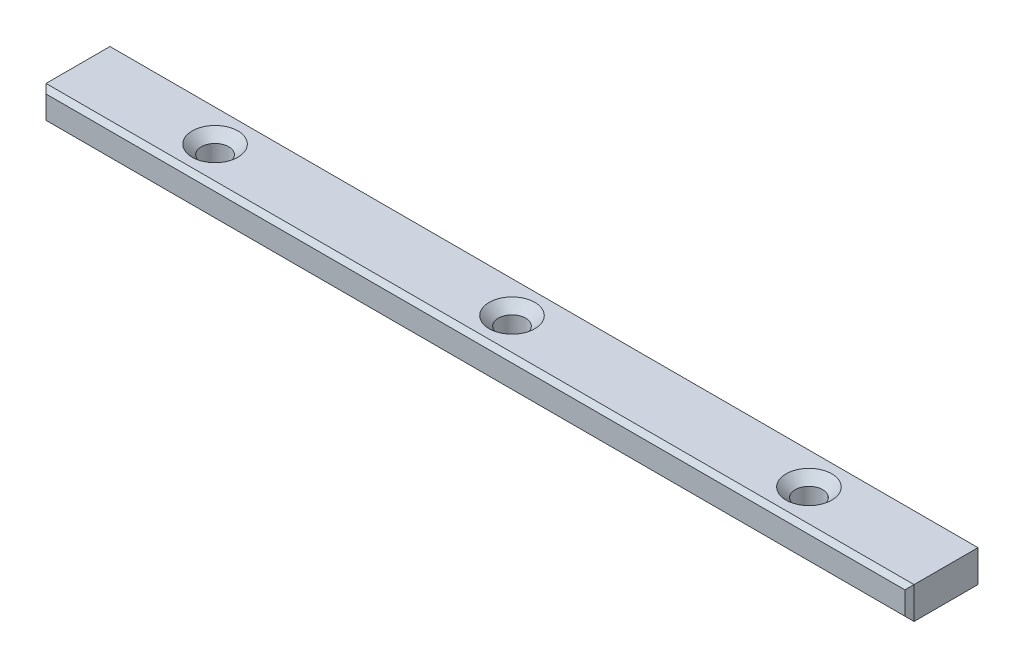
SolidWorks part; units mm, degrees
ref_plane "Front Plane" through (0, 0, 0) normal (0, 0, 1) x (1, 0, 0)
ref_plane "Top Plane" through (0, 0, 0) normal (0, 1, 0) x (1, 0, 0)
ref_plane "Right Plane" through (0, 0, 0) normal (1, 0, 0) x (0, 0, -1)
other "Configuration Table"
sketch "Sketch1" plane through (0, 0, 0) normal (0, 1, 0) x (1, 0, 0)
  line L1 (-95, 8) -> (95, 8)
  line L2 (-95, 8) -> (-95, -8)
  line L3 (-95, -8) -> (95, -8)
  line L4 (95, 8) -> (95, -8)
  line L5 (-95, 8) -> (95, -8) construction
  line L6 (-95, -8) -> (95, 8) construction
  point P0 (0, 0)
  dimension "D1" = 16
  dimension "D2" = 190
extrude "Boss-Extrude1" add sketch "Sketch1" along normal mid plane 7
sketch "Sketch2" plane through (0, 3.5, 0) normal (0, 1, 0) x (1, 0, 0)
  line L0 (-65, 0) -> (0, 0) construction
  line L1 (0, 0) -> (65, 0) construction
  point P0 (-65, 0)
  point P1 (0, 0)
  point P4 (65, 0)
  dimension "D1" = 65
  dimension "D2" = 65
hole_wizard "Hole1" positions "Sketch2" profile "Sketch3" legacy
sketch "Sketch3" plane through (-65, 3.5, 0) normal (1, 0, 0) x (0, 0, 1)
  line L0 (0, 0) -> (0, 20)
  line L1 (0, 20) -> (3, 20)
  line L2 (3, 20) -> (3, 2)
  line L3 (3, 2) -> (5, 0)
  line L4 (5, 0) -> (0, 0)
  line L5 (0, -6.4453) -> (0, 115.525) construction
  line L6 (-3, 2) -> (-5, 0) construction
  dimension "直径" = 6
  dimension "深度" = 20
  dimension "锥坑角度" = 90
  dimension "锥坑直径" = 10
chamfer "Chamfer1" distance 1 angle 45 8 edges at (95, 0, -8) (0, 3.5, -8) (-95, 0, -8) (0, -3.5, -8) (-95, 0, 8) (0, 3.5, 8) (95, 0, 8) (0, -3.5, 8)
